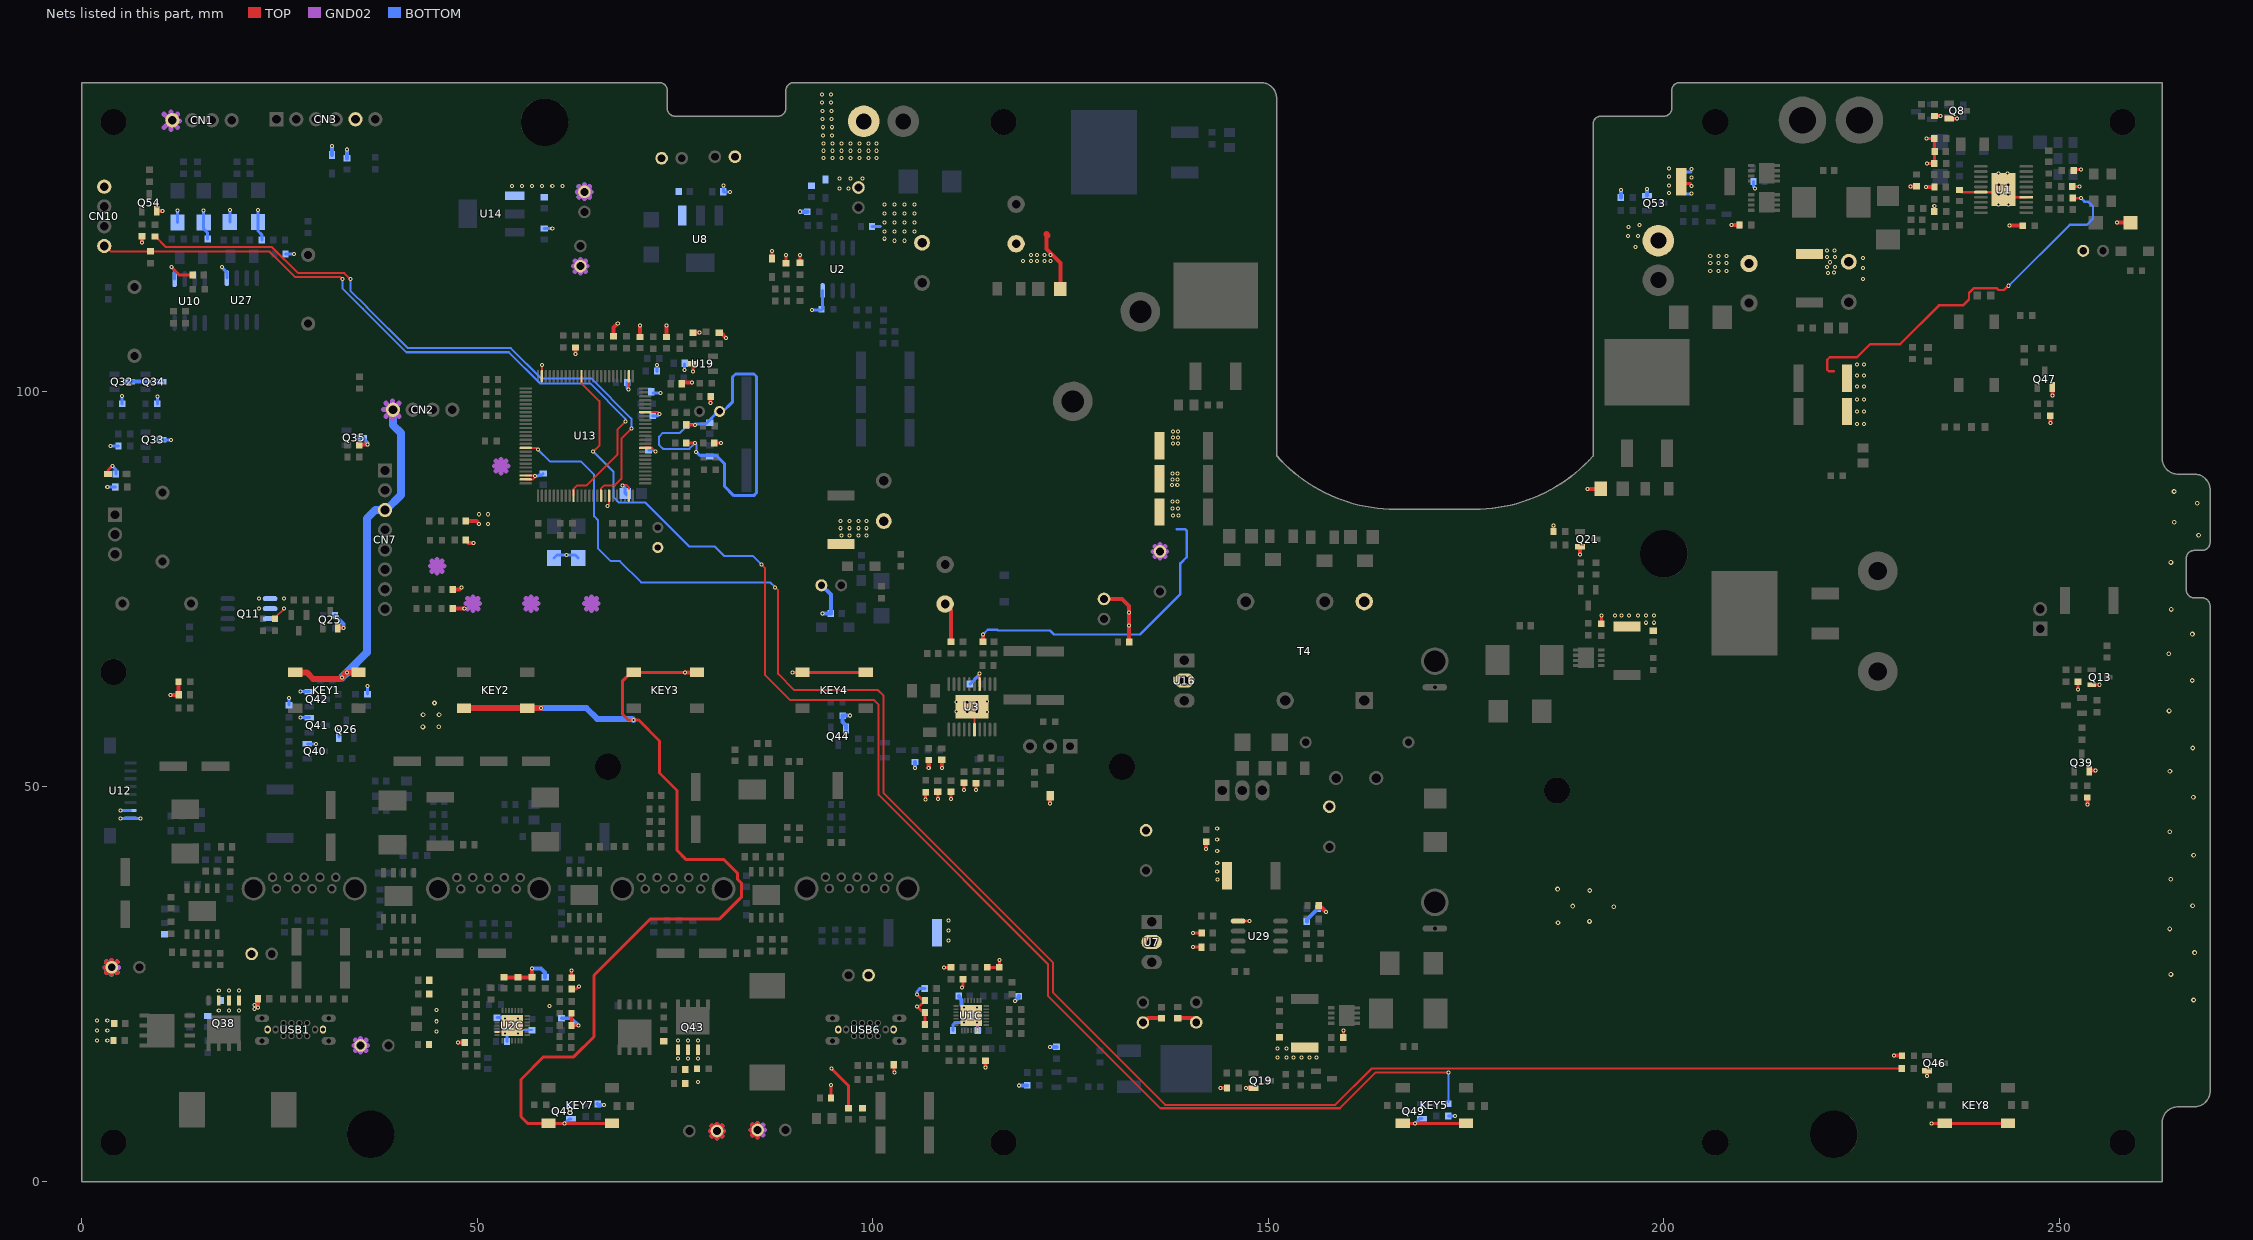
[diagram p0: the nets of this part, all layers, seen from the top]
# Altium PCB MISC84402.PcbDoc (part 5 of 12)
Units mm, origin at the board's own origin, x right, y up, seen from the top; angles counter-clockwise.
Board outline 269.06 x 139 mm, 4 copper layers (TOP, GND02, PWR03, BOTTOM), stack 0.732 mm thick; 694 components, 428 nets, 1859 pads, 1384 vias.

## Via types
v1: diameter 0.508, hole 0.254, TOP to BOTTOM, tented both sides, 1015 vias
v2: diameter 0.508, hole 0.254, TOP to BOTTOM, 243 vias
v3: diameter 0.508, hole 0.305, TOP to BOTTOM, 60 vias
v4: diameter 0.61, hole 0.305, TOP to BOTTOM, 55 vias
v5: diameter 0.61, hole 0.305, TOP to BOTTOM, tented both sides, 8 vias
v6: diameter 0.762, hole 0.381, TOP to BOTTOM, 2 vias
v7: diameter 0.762, hole 0.381, TOP to BOTTOM, tented both sides, 1 vias

## Nets (pads, with @x,y where several pads share a name; then routed paths per layer and width w, separated by ;. In a path a pad name is that pad's centre, name@x,y a point inside that pad or via, vN(x,y) a via of type N, cw(c..) or ccw(c..) an arc to the next point about the centre after c; other vN are vias at no path point) (continued)
GND: C1.2 C2.1 C4.2 C5.2 C6.2 C9.1 C11.1 C12.1 C13.2 C15.2 C21.1 C22.2 C25.1 C26.2 C27.1 C28.2 C30.2 C32.1 C34.1 C35.1 C36.1 C37.2 C38.2 C39.1 C40.1 C42.1 C43.1 C44.2 C45.2 C51.1 C52.2 C53.1 C54.2 C55.1 C56.1 C59.1 C61.1 C65.2 C69.1 C70.2 C71.1 C72.1 C73.2 C74.2 C75.2 C76.2 C78.1 C79.1 C83.1 C84.1 C85.1 C87.2 C88.1 C89.2 C90.1 C93.1 C94.2 C96.2 C97.2 C99.1 C100.1 C103.1 C107.2 C108.2 C109.2 C110.2 C111.2 C112.2 C113.1 C115.2 C116.2 C118.2 C119.1 C120.1 C121.1 C124.2 C125.2 C126.1 C127.1 C128.2 C129.1 C131.1 C132.2 C133.1 C134.2 C135.2 C136.1 C137.1 C138.1 C139.1 C140.2 C141.1 C146.2 C149.1 C152.2 C156.2 C159.2 C163.1 C164.1 C167.2 C168.1 C171.2 C176.1 C178.2 C179.1 C188.2 C189.2 C190.2 C191.2 C194.2 C399.1 CN1.1 CN2.4 CN3.5 CN7.3 CN10.4 D11.2 D12.2 D41.2 D42.2 D43.2 D44.2 D45.2 D46.1 D47.1 D48.2 D52.2 D57.2 J1.2 J13.2 KEY1.1 KEY1.2 KEY2.3 KEY2.4 KEY3.1 KEY3.2 KEY4.1 KEY4.2 KEY5.3 KEY5.4 KEY7.3 KEY7.4 KEY8.3 KEY8.4 Q8.2 Q11.1 Q11.2 Q11.3 Q13.2 Q19.2 Q21.2 Q25.2 Q26.2 Q32.3 Q33.3 Q34.3 Q35.3 Q38.1 Q38.2 Q38.3 Q39.2 Q40.2 Q41.2 Q42.2 Q43.1 Q43.2 Q43.3 Q44.2 Q46.2 Q47.2 Q48.2 Q49.2 Q53.2 Q54.2 R4.1 R5.1 R10.1 R11.1 R12.1 R14.2 R15.1 R18.1 R19.1 R21.2 R22.1 R26.1 R27.1 R41.1 R43.2 R44.2 R45.1 R51.1 R53.2 R55.1 R56.1 R57.1 R59.1 R65.2 R68.1 R72.2 R80.1 R88.2 R91.1 R93.1 R95.1 R105.1 R107.1 R110.1 R119.2 R122.2 R131.2 R145.1 R146.1 R161.2 R162.2 R163.2 R172.1 R177.2 R180.1 R181.2 R182.2 R183.1 R185.2 R190.2 R192.2 R193.2 R196.2 R209.2 R218.2 R223.1 R224.2 R227.1 R230.2 R265.1 R271.2 R272.2 R276.1 R296.1 R297.2 R306.2 R307.1 R309.1 R316.1 R321.2 R323.2 R332.2 R334.2 R336.2 R338.1 R350.1 R358.1 R365.2 R367.1 T4.8 U1.6 U1.14 U1.21 U1C.13 U1C.29 U2.4 U2C.13 U2C.29 U3.6 U3.14 U3.21 U7.2 U8.1 U10.5 U12.7 U12.8 U13.10 U13.19 U13.27 U13.49 U13.73 U13.74 U13.94 U13.99 U14.1 U16.2 U19.2 U27.5 U29.5 USB1.A1 USB1.A12 USB6.A1 USB6.A12 | length 738.2
  TOP w0.203: U2C.13@52.474,18.977 U2C.29@53.277,18.977 ; U1C.13@113.221,19.139 U1C.29@113.221,20.12
  TOP w0.254: R183.1@24.401,71.212 24.401,71.33 v1(25.553,72.482) ; U2C.29@53.277,18.977 v1(53.493,18.761) ; U13.74@56.103,88.826 57.049,88.826 57.303,89.08 v1(57.303,89.246) 57.223,89.326 U13.73@56.103,89.326 ; U13.49@58.153,101.876 v1(58.153,103.304) ; v1(66.421,85.471) 66.653,85.703 U13.94@66.653,86.776 ; v1@68.353,88.103 68.86,88.103 69.153,87.81 U13.99@69.153,86.776 ; v1(69.114,100.168) 69.153,100.207 U13.27@69.153,101.876 ; U13.19@71.203,97.326 72.845,97.326 v1(73.051,97.12) ; U3.6@112.847,57.198 U3.21@112.847,59.196 ; v1(113.183,20.158) 113.221,20.12 U1C.29@113.494,19.847 ; U3.14@113.497,62.944 v1@113.497,64.303
  TOP w0.305: U13.10@71.203,92.826 72.02,92.826 v1(72.517,92.329) ; U3.21@112.847,59.196 v5(113.122,59.471) ; v5(113.122,60.671) U3.21@113.497,61.046 ; 221.488,102.489 220.853,102.489 220.659,102.683 220.659,103.946 220.98,104.267 224.409,104.267 226.06,105.918 229.87,105.918 234.772,110.82 237.81,110.82 238.582,111.592 238.582,112.395 239.166,112.979 242.113,112.979 242.316,112.776 243.002,112.776 v1@243.51,113.284 ; C194.2@237.363,125.414 237.626,125.151 U1.6@240.078,125.151 242.076,125.151 v5(242.351,124.876) ; v5(243.551,124.876) 243.926,124.501 U1.14@245.824,124.501 ; R27.1@251.696,124.398 v1(252.73,124.398)
  TOP w0.381: D57.2@3.298,89.5 3.298,89.978 v1(3.836,90.516) ; v1(11.329,115.662) 12.345,114.646 C118.2@13.996,114.646 ; R185.2@61.901,21.328 R182.2@61.901,19.804 v1(62.798,19.804) ; R307.1@61.909,25.823 v1(61.909,26.712) ; R122.2@61.91,24.401 62.493,24.401 v1(62.823,24.731) ; KEY7.4@66.999,7.419 KEY7.3@58.999,7.419 56.335,7.419 55.499,8.255 55.499,12.954 58.367,15.822 62.177,15.822 64.727,18.372 64.727,26.119 71.882,33.274 80.636,33.274 83.414,36.052 83.414,37.735 82.906,38.243 82.906,39.005 81.169,40.742 76.42,40.742 75.235,41.926 75.235,49.505 73.025,51.714 73.025,55.753 70.383,58.395 v1@69.774,58.395 ; v1@69.774,58.42 v1(69.723,58.42) 69.079,58.42 68.326,59.173 68.326,63.312 69.433,64.419 v1(76.252,64.419) ; C164.1@76.418,93.437 v1(77.496,93.437) ; C127.1@76.418,95.723 v1(77.496,95.723) ; v1(77.262,102.454) U19.2@77.262,103.47 ; C126.1@79.974,93.437 v1(80.798,93.437) ; D41.2@87.249,116.743 v1(87.249,117.729) ; C159.2@89,116.143 v1(89,117.221) ; v2(89.809,64.419) KEY4.1@91.099,64.419 KEY4.2@99.099,64.419 ; R107.1@90.805,116.196 v1(90.805,117.221) ; C113.1@94.706,10.633 v1(94.706,12.284) ; v1(94.742,14.351) 96.901,12.192 C84.1@96.901,9.336 ; C88.1@102.639,14.824 102.639,13.947 v1(102.743,13.843) ; v1(105.563,23.714) 106.325,22.952 C135.2@106.579,22.952 105.817,22.19 v1(105.563,22.19) 106.325,21.428 C108.2@106.579,21.428 C146.2@106.579,19.904 ; v1(106.68,48.387) R11.1@106.68,49.285 ; v1(108.204,48.44) C42.1@108.204,49.338 ; v1(108.992,27.142) R309.1@109.881,27.143 ; v1(109.855,48.44) C12.1@109.855,49.338 ; v1(111.278,24.603) 111.405,24.73 R196.2@111.405,25.619 ; v1(111.506,49.583) C13.2@111.506,50.481 ; v1(113.03,49.53) R14.2@113.03,50.428 ; R161.2@114.453,27.125 R162.2@115.977,27.125 v1(115.977,28.041) ; v1(140.488,29.683) C45.2@141.55,29.683 C45.2@141.566,29.683 ; v1(140.488,31.461) C40.1@141.566,31.461 ; U29.5@146.172,32.985 v1(147.6,32.985) ; R72.2@159.475,18.253 v1(159.475,19.14) ; KEY5.3@167,7.419 KEY5.4@175,7.419 ; R172.1@192.095,70.568 v1(192.095,71.593) ; R26.1@202.145,126.242 203.399,126.242 ; v2(233.198,131.927) R12.1@234.197,131.927 R10.1@234.197,128.749 ; v1(233.299,128.749) R10.1@234.197,128.749 ; v2@233.814,7.42 v2(233.83,7.42) ; v2@233.814,7.42 KEY8.4@243.5,7.42 ; R306.2@234.197,122.682 v1@234.197,123.393 ; R10.1@234.25,128.802 R10.1@234.197,128.749 ; C27.1@251.652,125.857 v1(252.55,125.857) ; R55.1@251.823,128.016 v1(252.721,128.016) ; v1(252.375,62.291) R68.1@252.375,63.258 ; Q13.2@254.102,62.865 v1(255.103,62.865)
  TOP w0.508: v2(7.585,118.754) R365.2@7.585,119.55 ; Q54.2@9.476,122.791 v2(10.204,122.791) ; v1(11.176,61.595) C168.1@12.254,61.595 12.201,61.648 R321.2@12.201,63.246 ; v2(22.262,22.084) C141.1@22.262,23.165 ; Q25.2@32.36,70.069 v2(33.081,70.069) ; R146.1@35.061,93.183 35.113,93.235 v1(36.128,93.235) ; C72.1@46.866,72.517 v2(48.336,72.517) ; C71.1@46.866,74.93 47.752,74.93 v1(48.006,75.184) ; v2(47.533,17.638) R218.2@48.412,17.638 ; C59.1@48.514,83.566 49.861,83.566 v1(50.225,83.202) ; C69.1@48.517,81.153 48.898,80.772 v1(49.53,80.772) ; C134.2@53.366,25.875 C111.2@56.922,25.875 v1(56.922,27.016) ; v1(62.383,104.674) R224.2@62.383,105.51 ; C100.1@67.199,106.906 67.199,108.017 v2(67.742,108.56) ; C99.1@70.552,106.829 v2(70.552,108.296) ; C21.1@73.889,106.821 v2(73.889,108.306) ; C35.1@75.841,100.923 75.985,101.067 v2(77.114,101.067) ; v1(76.252,64.419) KEY3.2@77.763,64.419 ; C34.1@77.232,107.388 v2(78.057,107.388) ; v2(79.481,98.472) C5.2@79.481,99.314 ; C26.2@80.568,107.37 80.793,107.37 v2(81.432,106.731) ; v1(107.061,52.324) R223.1@107.061,53.349 ; v1(108.712,52.324) C15.2@108.712,53.402 ; C171.2@109.133,73.065 109.855,72.343 R15.1@109.855,68.317 ; R22.1@113.919,68.317 v1(113.919,69.215) ; v2(114.223,14.453) R181.2@114.223,15.344 ; 121.92,119.819 121.92,117.983 123.701,116.202 C25.1@123.701,112.903 ; v2(122.403,47.829) D48.2@122.403,48.838 ; C65.2@129.218,73.711 131.478,73.711 132.393,72.796 v1(132.393,72.009) v1(132.393,70.358) C96.2@132.393,68.25 ; C30.2@134.315,20.218 134.799,20.702 C28.2@136.51,20.702 ; C167.2@138.547,20.713 140.399,20.713 C76.2@140.792,20.32 ; v1(142.139,42.129) R265.1@142.139,43.026 ; v2(143.968,11.887) R65.2@144.762,11.887 ; v2(147.166,11.86) Q19.2@148.114,11.86 ; C89.2@156.354,34.976 156.472,34.976 v1(157.285,34.163) ; R44.2@186.042,82.219 v2(186.042,82.969) ; v2(189.389,79.343) Q21.2@189.389,80.313 ; v1(190.356,87.63) C36.1@192.004,87.63 ; v2(208.559,120.98) R56.1@209.559,120.98 ; v2(229.099,15.96) R323.2@230.116,15.96 ; v2(231.182,125.866) R296.1@231.927,125.866 ; v2(233.172,125.806) C37.2@234.225,125.806 ; v2(233.281,13.393) Q46.2@233.281,14.07 ; R297.2@234.204,134.764 v2(234.993,134.764) ; Q8.2@236.084,134.457 v2(237.048,134.457) ; v1(243.713,120.904) R21.2@245.373,120.904 ; v2(248.86,95.97) R332.2@248.86,96.867 ; v2(249.125,99.465) Q47.2@249.125,100.489 ; v2(253.534,47.736) R272.2@253.534,48.607 ; Q39.2@253.799,52.026 v2(254.591,52.026) ; v1(257.302,121.285) D52.2@258.986,121.285
  TOP w0.635: 2.913,27.143 C140.2@3.765,27.143 ; 3.112,26.49 C140.2@3.765,27.143 ; 3.112,27.795 C140.2@3.765,27.143 ; 3.765,26.291 C140.2@3.765,27.143 ; 3.765,27.994 C140.2@3.765,27.143 ; 4.418,26.49 C140.2@3.765,27.143 ; 4.418,27.795 C140.2@3.765,27.143 ; 79.438,6.442 C97.2@80.29,6.442 ; 79.637,5.789 C97.2@80.29,6.442 ; 79.637,7.094 C97.2@80.29,6.442 ; 80.29,5.59 C97.2@80.29,6.442 ; 80.29,7.293 C97.2@80.29,6.442 ; 80.943,5.789 C97.2@80.29,6.442 ; 80.943,7.094 C97.2@80.29,6.442 ; 81.141,6.442 C97.2@80.29,6.442 ; 84.574,6.569 C107.2@85.426,6.569 ; 84.773,5.916 C107.2@85.426,6.569 ; 84.773,7.221 C107.2@85.426,6.569 ; 85.426,5.717 C107.2@85.426,6.569 ; 85.426,7.42 C107.2@85.426,6.569
  TOP w0.762: KEY1.1@26.964,64.419 28.408,64.419 29.236,63.592 32.665,63.592 v1(32.854,63.781) v1(33.492,64.419) KEY1.2@34.964,64.419 ; KEY2.3@48.3,59.919 KEY2.4@56.3,59.919 v1(58.039,59.92) ; 121.92,119.819 122.05,119.689
  GND02 w0.635: 2.913,27.143 C140.2@3.765,27.143 ; 3.112,26.49 C140.2@3.765,27.143 ; 3.112,27.795 C140.2@3.765,27.143 ; 3.765,26.291 C140.2@3.765,27.143 ; 3.765,27.994 C140.2@3.765,27.143 ; 4.418,26.49 C140.2@3.765,27.143 ; 4.418,27.795 C140.2@3.765,27.143 ; 4.616,27.143 C140.2@3.765,27.143 ; 10.403,133.333 CN1.1@11.233,134.163 ; 10.403,134.992 CN1.1@11.233,134.163 ; 11.233,133.062 CN1.1@11.233,134.163 ; 11.233,135.264 CN1.1@11.233,134.163 ; 12.062,133.333 CN1.1@11.233,134.163 ; 12.062,134.992 CN1.1@11.233,134.163 ; 12.334,134.163 CN1.1@11.233,134.163 ; 34.381,17.265 C115.2@35.233,17.265 ; 34.58,16.612 C115.2@35.233,17.265 ; 34.58,17.917 C115.2@35.233,17.265 ; 35.233,16.413 C115.2@35.233,17.265 ; 35.233,18.116 C115.2@35.233,17.265 ; 35.886,16.612 C115.2@35.233,17.265 ; 35.886,17.917 C115.2@35.233,17.265 ; 36.084,17.265 C115.2@35.233,17.265 ; 38.147,97.638 CN2.4@39.249,97.638 ; 38.419,96.808 CN2.4@39.249,97.638 ; 38.419,98.467 CN2.4@39.249,97.638 ; 39.249,96.536 CN2.4@39.249,97.638 ; 39.249,98.739 CN2.4@39.249,97.638 ; 40.078,96.808 CN2.4@39.249,97.638 ; 40.078,98.467 CN2.4@39.249,97.638 ; 44.04,77.868 44.891,77.868 ; 44.238,77.215 44.891,77.868 ; 44.238,78.521 44.891,77.868 ; 44.891,77.017 44.891,77.868 ; 44.891,78.719 44.891,77.868 ; 45.544,77.215 44.891,77.868 ; 45.544,78.521 44.891,77.868 ; 45.742,77.868 44.891,77.868 ; 48.578,73.117 49.429,73.117 ; 48.776,72.464 49.429,73.117 ; 48.776,73.769 49.429,73.117 ; 49.429,72.265 49.429,73.117 ; 49.429,73.968 49.429,73.117 ; 50.082,72.464 49.429,73.117 ; 50.082,73.769 49.429,73.117 ; 50.28,73.117 49.429,73.117 ; 52.133,90.516 52.985,90.516 ; 52.332,89.863 52.985,90.516 ; 52.332,91.168 52.985,90.516 ; 52.985,89.664 52.985,90.516 ; 52.985,91.367 52.985,90.516 ; 53.638,89.863 52.985,90.516 ; 53.638,91.168 52.985,90.516 ; 53.836,90.516 52.985,90.516 ; 55.944,73.117 56.795,73.117 ; 56.142,72.464 56.795,73.117 ; 56.142,73.769 56.795,73.117 ; 56.795,72.265 56.795,73.117 ; 56.795,73.968 56.795,73.117 ; 57.448,72.464 56.795,73.117 ; 57.448,73.769 56.795,73.117 ; 57.646,73.117 56.795,73.117 ; 62.166,115.789 C152.2@63.018,115.789 ; 62.365,115.136 C152.2@63.018,115.789 ; 62.365,116.441 C152.2@63.018,115.789 ; 62.674,125.187 C156.2@63.526,125.187 ; 62.873,124.534 C156.2@63.526,125.187 ; 62.873,125.839 C156.2@63.526,125.187 ; 63.018,114.937 C152.2@63.018,115.789 ; 63.018,116.64 C152.2@63.018,115.789 ; 63.526,124.335 C156.2@63.526,125.187 ; 63.526,126.038 C156.2@63.526,125.187 ; 63.563,73.117 64.415,73.117 ; 63.671,115.136 C152.2@63.018,115.789 ; 63.671,116.441 C152.2@63.018,115.789 ; 63.762,72.464 64.415,73.117 ; 63.762,73.769 64.415,73.117 ; 63.869,115.789 C152.2@63.018,115.789 ; 64.179,124.534 C156.2@63.526,125.187 ; 64.179,125.839 C156.2@63.526,125.187 ; 64.377,125.187 C156.2@63.526,125.187 ; 64.415,72.265 64.415,73.117 ; 64.415,73.968 64.415,73.117 ; 65.068,72.464 64.415,73.117 ; 65.068,73.769 64.415,73.117 ; 65.266,73.117 64.415,73.117 ; 79.438,6.442 C97.2@80.29,6.442 ; 79.637,5.789 C97.2@80.29,6.442 ; 79.637,7.094 C97.2@80.29,6.442 ; 80.29,5.59 C97.2@80.29,6.442 ; 80.29,7.293 C97.2@80.29,6.442 ; 80.943,5.789 C97.2@80.29,6.442 ; 80.943,7.094 C97.2@80.29,6.442 ; 81.141,6.442 C97.2@80.29,6.442 ; 84.574,6.569 C107.2@85.426,6.569 ; 84.773,5.916 C107.2@85.426,6.569 ; 84.773,7.221 C107.2@85.426,6.569 ; 85.426,5.717 C107.2@85.426,6.569 ; 85.426,7.42 C107.2@85.426,6.569 ; 86.079,5.916 C107.2@85.426,6.569 ; 86.079,7.221 C107.2@85.426,6.569 ; 86.277,6.569 C107.2@85.426,6.569 ; 135.445,79.721 C116.2@136.297,79.721 ; 135.644,79.068 C116.2@136.297,79.721 ; 135.644,80.373 C116.2@136.297,79.721 ; 136.297,78.869 C116.2@136.297,79.721 ; 136.297,80.572 C116.2@136.297,79.721 ; 136.95,79.068 C116.2@136.297,79.721 ; 136.95,80.373 C116.2@136.297,79.721 ; 137.148,79.721 C116.2@136.297,79.721
  BOTTOM w0.254: v1(55.144,18.761) 55.587,19.204 C103.1@56.922,19.204 ; C74.2@76.384,95.742 76.384,95.484 75.616,94.717 73.457,94.717 72.974,94.234 72.974,93.193 73.051,93.116 73.051,93.099 73.466,92.685 76.784,92.685 v1@77.445,93.345 ; v1(77.496,93.437) 77.673,93.259 v2@77.673,92.456
  BOTTOM w0.305: C137.1@71.628,92.518 72.328,92.518 v1(72.517,92.329) ; v1(113.919,69.215) 114.529,69.825 115.722,69.825 115.824,69.723 122.384,69.723 122.892,69.215 133.775,69.215 138.884,74.324 138.884,78.203 139.675,78.994 ; 138.43,82.55 139.446,82.55 139.7,82.296 139.7,78.994 ; v1(243.586,113.309) 243.611,113.309 251.333,121.031 253.492,121.031 254.254,121.793 254.254,123.317 253.619,123.952 253.176,123.952 v1(252.73,124.398)
  BOTTOM w0.381: v1(3.201,87.849) R276.1@4.226,87.849 ; v1(3.582,93.073) R105.1@4.598,93.073 ; v1(3.836,90.516) 4.279,90.072 C93.1@4.279,89.5 ; v2(4.846,45.979) U12.8@6.126,45.979 v2(7.422,45.979) ; v2(4.862,46.979) U12.7@6.126,46.979 ; R91.1@5.088,98.39 v1(5.088,99.388) ; R93.1@9.542,98.39 v1(9.542,99.279) ; Q33.3@10.043,93.818 v1(11.272,93.818) ; v1(11.329,115.662) 11.71,115.281 U10.5@11.71,114.138 ; D42.2@12.091,121.314 v1(12.091,122.838) ; v1(15.393,122.838) 15.393,120.488 15.901,119.98 R192.2@15.901,119.218 ; v1(17.679,115.662) 18.314,115.027 U27.5@18.314,114.265 ; D45.2@18.695,121.377 v1(18.695,122.901) ; v1(22.251,122.901) 22.251,120.234 22.741,119.743 R230.2@22.741,119.091 ; C124.2@25.745,117.313 v1(26.823,117.313) ; R180.1@26.188,60.281 v1(26.188,61.179) ; v1(27.617,58.7) Q41.2@28.74,58.7 ; v1(27.617,62.002) Q42.2@28.74,62.002 ; Q40.2@28.49,55.398 v1(29.613,55.398) ; Q26.2@32.477,56.242 v1(32.477,57.364) ; R95.1@36.094,61.678 v1(36.094,62.703) ; C121.1@52.474,20.777 53.382,20.776 v1(53.493,20.666) ; v1(53.493,18.761) 53.749,18.504 C136.1@53.749,17.745 ; v1(57.303,89.246) 57.684,89.246 57.811,89.373 58.127,89.373 C131.1@58.319,89.565 ; C9.1@58.446,120.553 v1(59.462,120.552) ; D46.1@59.69,78.899 60.068,79.277 v1(61.24,79.277) 62.36,79.277 D47.1@62.738,78.899 ; R88.2@60.639,20.7 61.901,20.7 v1(62.798,19.804) ; v2(60.985,7.391) 61.568,7.974 Q48.2@61.842,7.974 ; 68.562,87.84 68.631,87.771 C178.2@68.631,87.02 ; C178.2@68.86,86.833 C178.2@68.86,87.03 ; C133.1@68.925,101.057 68.925,100.357 v1(69.114,100.168) ; R80.1@72.153,96.866 72.797,96.866 v1(73.051,97.12) ; C39.1@72.177,99.731 v1(73.128,99.731) ; C73.2@72.701,102.498 v2(72.701,103.271) ; v2(76.155,102.661) C52.2@76.155,103.438 ; C74.2@76.384,95.742 v1@77.435,95.742 ; v1@77.521,95.834 78.867,95.834 79.731,96.698 79.731,96.728 80.259,97.257 R163.2@80.899,97.257 ; v2(77.656,92.311) 78.121,91.846 80.196,91.846 81.229,90.813 81.229,88.722 ; R163.2@80.924,97.282 82.22,98.577 82.22,101.727 82.446,101.953 ; v2(81.099,126.006) C78.1@81.099,125.187 v2(81.924,125.187) ; 81.229,88.494 81.229,88.722 ; 82.446,101.954 82.632,102.14 84.982,102.14 85.293,101.829 85.293,87.122 84.938,86.766 82.423,86.766 81.229,87.96 81.229,88.722 ; v1(92.329,110.236) 93.488,110.236 93.649,110.397 U2.4@93.649,112.677 ; C54.2@99.887,120.777 100.965,120.777 ; v1(105.563,23.714) 105.563,24.095 105.944,24.476 C110.2@106.576,24.476 ; C179.1@110.135,19.142 110.135,19.904 110.389,20.158 v1(111.532,20.158) ; R43.2@112.268,62.941 113.462,64.135 v1@113.462,64.287 ; v1(113.183,20.158) 113.245,20.095 C120.1@113.245,19.142 ; v2(168.529,7.391) 169.137,7.999 Q49.2@169.411,7.999 ; R336.2@172.754,8.34 v2(173.618,8.34) ; v2@203.454,124.917 202.438,124.917 202.145,125.21 202.145,127.419 202.438,127.711 203.454,127.711 ; C51.1@211.325,126.502 211.325,125.805 v1(211.517,125.613)
  BOTTOM w0.508: Q32.3@6.096,101.184 v1(8.829,101.184) Q34.3@10.059,101.184 ; D11.2@31.623,129.853 v1(31.623,130.996) ; R193.2@31.996,71.644 33.071,70.568 v2@33.071,70.18 ; C2.1@33.528,129.416 v1(33.528,130.559) ; Q35.3@35.433,94.107 36.128,93.412 v1(36.128,93.235) ; v1(56.922,27.016) 58.065,27.016 58.573,26.508 C132.2@58.573,25.875 ; R334.2@65.21,9.864 65.321,9.754 v2(65.989,9.754) ; v2(90.796,122.666) R271.2@91.712,122.666 ; C191.2@93.492,75.438 94.677,74.253 C11.1@94.677,71.882 v1(93.599,71.882) ; R53.2@96.164,58.75 96.164,58.166 96.598,57.732 Q44.2@96.598,57.346 ; R53.2@96.181,58.953 v2(97.104,58.953) ; v2(105.308,52.324) R51.1@105.308,53.095 ; C22.2@110.856,23.505 110.856,23.383 111.227,23.012 111.227,22.377 v1@111.481,22.123 ; v2(117.958,22.86) 118.457,23.36 R119.2@118.457,23.485 ; v2(118.475,12.227) R350.1@119.507,12.227 ; v2(122.378,17.094) R338.1@123.199,17.094 ; R190.2@154.872,32.944 154.872,33.195 C70.2@156.272,34.595 156.853,34.595 v1(157.285,34.163) ; R177.2@194.554,124.45 v2(194.554,125.415) ; Q53.2@197.848,124.716 v2(197.848,125.534)
  BOTTOM w0.635: 3.112,26.49 C140.2@3.765,27.143 ; 3.112,27.795 C140.2@3.765,27.143 ; 3.765,26.291 C140.2@3.765,27.143 ; 3.765,27.994 C140.2@3.765,27.143 ; 4.418,26.49 C140.2@3.765,27.143 ; 4.418,27.795 C140.2@3.765,27.143 ; 4.616,27.143 C140.2@3.765,27.143 ; 62.674,125.187 C156.2@63.526,125.187 ; 62.873,124.534 C156.2@63.526,125.187 ; 62.873,125.839 C156.2@63.526,125.187 ; 63.526,124.335 C156.2@63.526,125.187 ; 63.526,126.038 C156.2@63.526,125.187 ; 64.179,124.534 C156.2@63.526,125.187 ; 64.179,125.839 C156.2@63.526,125.187 ; 64.377,125.187 C156.2@63.526,125.187
  BOTTOM w0.762: v1(58.039,59.92) 63.779,59.919 65.151,58.547 69.596,58.547 v1(69.723,58.42)
  BOTTOM w1.016: v1(32.854,63.781) v1(33.492,64.419) 36.015,66.941 36.015,83.883 37.119,84.987 38.465,84.987 40.333,86.855 40.333,94.678 39.329,95.682 CN2.4@39.329,97.638
  other v1: 77.877,12.665 75.337,15.586 76.607,15.586 77.877,15.586 151.156,15.713 152.299,15.713 153.188,15.713 154.204,15.713 155.22,15.713 156.109,15.713 151.156,16.856 152.299,16.856 1.931,17.872 3.201,17.872 75.337,17.872 76.607,17.872 77.877,17.872 44.831,19.05 1.931,19.142 3.201,19.142 54.382,19.777 44.831,20.32 1.931,20.412 3.201,20.412 55.144,20.666 112.421,21.174 17.298,21.682 18.568,21.682 19.838,21.682 44.831,21.717 111.532,22.063 113.183,22.063 59.14,22.267 17.298,24.222 18.568,24.222 19.838,24.222 109.551,30.546 109.551,31.816 109.551,33.086 143.561,38.242 143.536,39.284 143.536,40.351 143.536,41.875 143.536,43.272 143.536,44.669 114.416,59.447 110.566,59.487 110.555,60.692 114.416,60.717 113.486,64.314 197.765,70.704 198.781,70.704 193.853,71.593 194.641,71.593 195.606,71.593 196.749,71.593 197.765,71.593 198.781,71.593 22.378,72.482 22.378,73.752 25.553,73.752 96.012,81.763 97.053,81.763 98.196,81.763 99.212,81.763 95.91,82.652 97.053,82.652 98.196,82.652 99.212,82.652 51.368,83.202 95.91,83.541 97.053,83.541 98.196,83.541 99.212,83.541 50.225,84.421 51.368,84.421 137.897,86.004 138.532,86.004 68.326,88.076 137.846,88.113 138.481,88.113 137.854,88.8 138.489,88.8 137.854,89.562 138.489,89.562 137.922,93.345 138.557,93.345 137.936,94.107 138.571,94.107 137.936,94.869 138.571,94.869 224.392,95.833 225.281,95.833 224.41,97.409 225.299,97.409 224.392,98.933 225.281,98.933 224.392,100.584 225.281,100.584 224.392,101.981 225.281,101.981 224.392,103.378 225.281,103.378 225.171,114.173 220.751,114.935 221.488,114.986 205.867,115.189 206.883,115.189 207.899,115.189 225.171,115.57 220.599,115.697 221.615,115.697 205.867,116.205 206.883,116.205 207.899,116.205 221.031,116.281 118.999,116.459 120.015,116.459 120.777,116.459 121.666,116.459 122.428,116.459 225.171,116.84 220.599,116.967 221.615,116.967 205.867,117.094 206.883,117.094 207.899,117.094 120.015,117.221 120.777,117.221 121.666,117.221 122.428,117.221 220.599,117.78 221.59,117.78 196.444,118.212 102.743,118.999 104.013,118.999 101.473,119.253 195.478,119.583 196.748,119.609 101.473,120.142 102.743,120.142 104.013,120.142 105.283,120.142 195.555,120.752 196.926,121.006 101.473,121.285 102.743,121.285 104.013,121.285 105.283,121.285 101.473,122.428 102.743,122.428 104.013,122.428 105.283,122.428 234.188,123.419 101.473,123.571 102.743,123.571 104.013,123.571 105.283,123.571 242.316,123.571 243.586,123.571 95.758,125.603 96.901,125.603 203.505,125.908 54.382,125.949 55.652,125.949 56.922,125.949 58.192,125.949 59.462,125.949 60.732,125.949 95.758,126.873 97.155,126.873 98.679,126.873 203.475,126.979 242.316,127.508 243.459,127.508 200.635,128.118 93.73,129.489 94.873,129.489 96.016,129.489 97.159,129.489 98.302,129.489 99.445,129.489 100.461,129.489 93.73,130.378 94.873,130.378 96.016,130.378 97.159,130.378 98.302,130.378 99.445,130.378 100.461,130.378 93.73,131.267 94.873,131.267 96.016,131.267 97.159,131.267 98.302,131.267 99.445,131.267 100.461,131.267 93.701,132.309 94.844,132.309 93.671,133.35 94.814,133.35 93.642,134.391 94.785,134.391 93.613,135.433 94.756,135.433 93.584,136.474 94.727,136.474 93.555,137.516 94.698,137.516
  other v2: 21.844,21.869 21.793,22.403 137.922,84.252 138.608,84.252 137.897,85.166 138.557,85.166 203.505,124.943 200.66,125.044 200.66,126.009 200.66,127.102 203.479,128.092
  other v4: 266.979,23.012 264.109,26.238 267.106,29.007 263.957,32.004 186.614,32.766 190.602,32.944 193.675,34.798 188.493,34.874 266.852,34.925 190.627,36.855 186.563,37.033 264.084,38.278 266.979,41.3 263.957,44.272 266.954,48.641 263.982,51.918 266.878,54.864 43.104,57.531 45.11,57.556 43.129,59.08 45.161,59.08 263.881,59.563 44.577,60.554 266.802,63.398 263.83,66.777 266.827,69.266 264.16,72.39 264.109,78.334 267.614,81.763 264.541,83.414 267.437,85.801 264.516,87.3
  other v5: 111.922,59.471 111.922,60.671 242.351,126.076 243.551,126.076
KEY9-EN: R364.1 U13.92 | length 82.6
  TOP w0.254: R364.1@9.347,119.482 10.627,118.202 24.029,118.202 27.331,114.9 33.173,114.9 v1(33.935,114.138) ; U13.92@65.653,86.776 65.653,87.689 66.04,88.076 67.375,88.076 68.199,88.9 68.199,93.98 v1(69.469,95.25)
  BOTTOM w0.254: v1(33.935,114.138) 33.935,112.697 35.991,110.641 36.094,110.538 41.222,105.41 54.229,105.41 58.039,101.6 64.389,101.6 69.469,96.52 v1(69.469,95.25)
KEY9-MCU: CN10.1 R366.1 U13.85 | length 91.9
  TOP w0.254: CN10.1@3.226,118.11 3.708,117.627 23.714,117.627 24.951,116.391 26.95,114.392 32.665,114.392 v1(32.919,114.138) ; U13.85@62.153,86.776 62.153,87.617 62.611,88.076 63.819,88.076 67.691,91.948 67.691,95.123 v1(68.707,96.139)
  BOTTOM w0.254: v1(32.919,114.138) 32.919,112.995 ; 35.505,110.409 32.919,112.995 ; v1(68.707,96.139) 68.707,96.52 64.262,100.965 57.912,100.965 53.975,104.902 41.012,104.902 32.919,112.995
KEY-DC: R337.1 U13.39 | length 177.8
  TOP w0.254: U13.39@63.153,101.876 63.153,100.982 65.405,98.73 65.405,93.091 64.668,92.354 v2(64.643,92.354) ; v2(85.903,78.08) 86.335,77.648 86.335,64.11 89.535,60.909 100.152,60.909 100.736,60.325 100.736,48.946 122.123,27.559 122.123,23.546 136.347,9.322 159.029,9.322 163.525,13.818 v2(172.745,13.818)
  BOTTOM w0.254: v2(64.643,92.354) 67.234,89.764 67.234,87.198 ; 67.234,87.02 67.234,87.198 ; v2(85.903,78.08) 84.811,79.172 81.178,79.172 80.01,80.34 76.784,80.34 71.222,85.903 67.894,85.903 67.234,86.563 67.234,87.198 ; R337.1@172.745,10.135 v2(172.745,13.818)
KEY-LED: R325.1 U13.66 | length 231
  TOP w0.254: U13.66@56.103,92.826 57.415,92.826 v1(57.658,92.583) ; v1(87.63,75.184) 88.011,74.803 88.011,64.235 90.016,62.23 100.584,62.23 101.346,61.468 101.346,49.149 122.784,27.711 122.784,23.927 136.957,9.754 158.471,9.754 163.068,14.351 R325.1@229.972,14.351
  BOTTOM w0.254: v1(57.658,92.583) 59.182,91.059 63.119,91.059 64.77,89.408 64.77,84.15 65.227,83.693 65.227,80.112 66.833,78.505 68.015,78.505 70.701,75.819 86.995,75.819 v1(87.63,75.184)